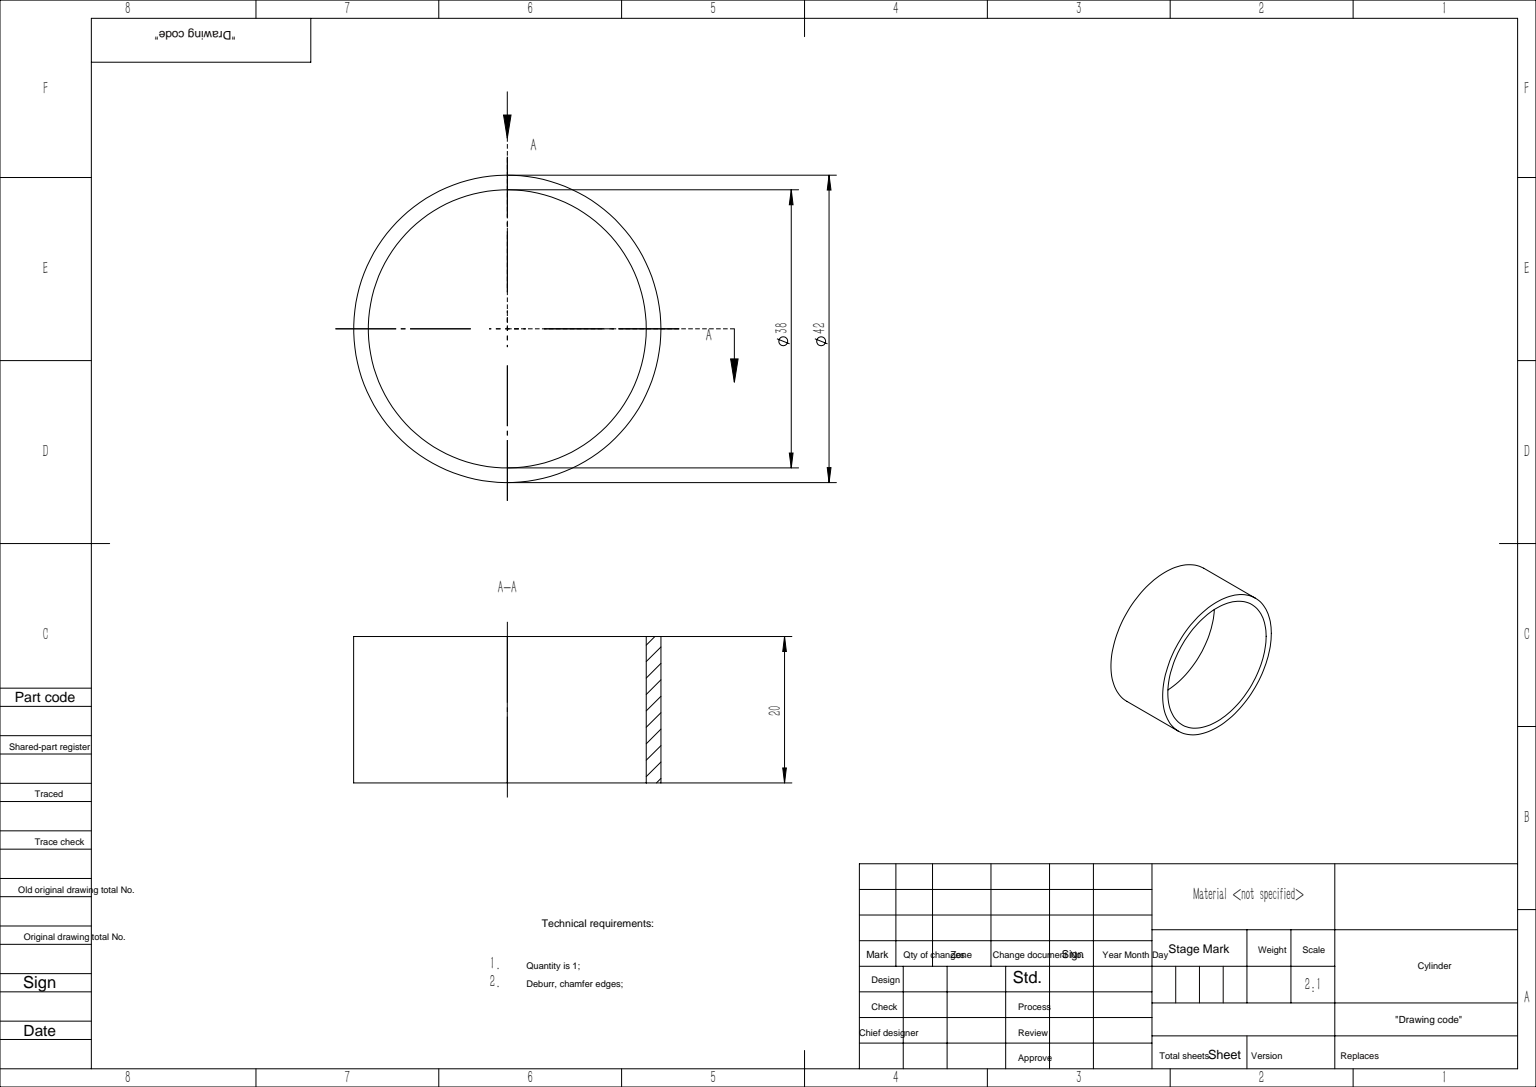
from build123d import *

# Parameters (mm, degrees)
SKETCH_1_R      = 21
SKETCH_1_R_2    = 19
EXTRUDE_1_DEPTH = 20


with BuildPart() as part:
    # 草图1 → 凸台-拉伸1 (new body)
    with BuildSketch(Plane(origin=(629.7, 0, 0), x_dir=(0, 0, -1), z_dir=(1, 0, 0))):
        with Locations((201, -379)):
            Circle(SKETCH_1_R)
        with Locations((201, -379)):
            Circle(SKETCH_1_R_2, mode=Mode.SUBTRACT)
    extrude(amount=EXTRUDE_1_DEPTH)


solid = part.part
